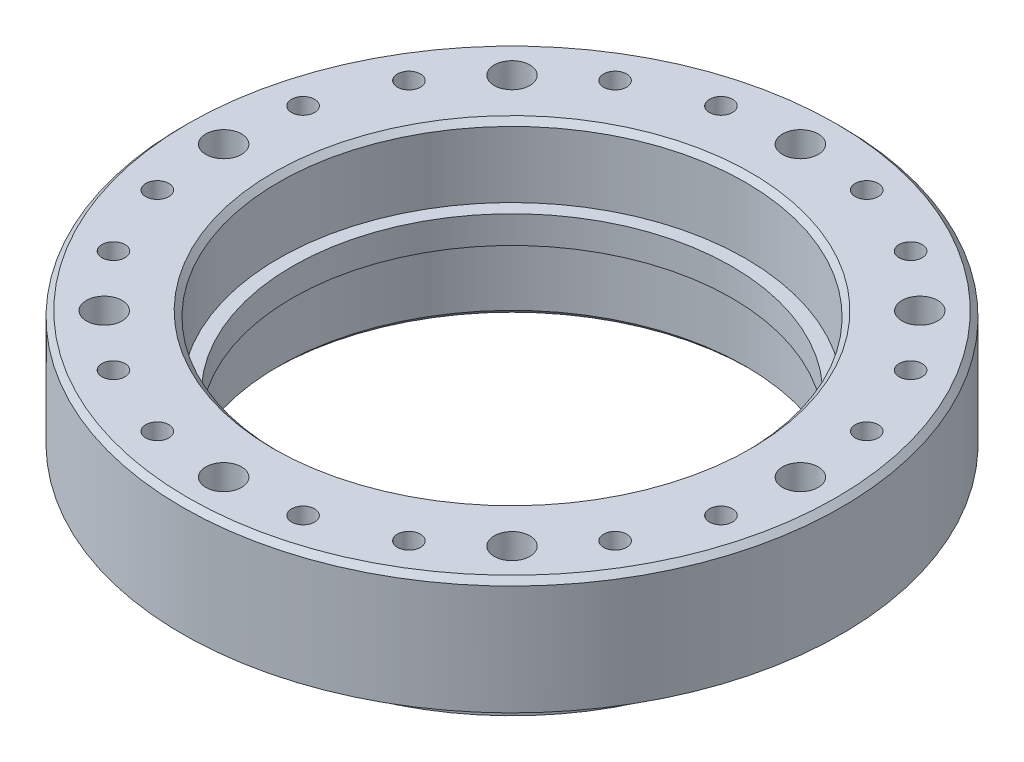
from build123d import *

# Parameters (mm, degrees)
SKETCH_1_R                = 60
SKETCH_1_R_2              = 40
EXTRUDE_1_DEPTH           = 15.5
CHAMFER_1_SIZE            = 1
HOLE_WIZARD_1_D           = 6.5
HOLE_WIZARD_1_CBORE_D     = 11
HOLE_WIZARD_1_CBORE_DEPTH = 6.8
SKETCH_7_R                = 42.5
CUT_EXTRUDE_2_DEPTH       = 13
CUT_EXTRUDE_START         = -13
SKETCH_8_R                = 42.5
CUT_EXTRUDE_3_DEPTH       = 13
SKETCH_9_R                = 67.994168063
SKETCH_9_R_2              = 46.5
CUT_EXTRUDE_4_DEPTH       = 10
HOLE_WIZARD_M5_1_D        = 4.2
PATTERN_CIRCULAR_1_COUNT  = 8
SKETCH_10_R               = 6
CUT_EXTRUDE_5_DEPTH       = 10
PATTERN_CIRCULAR_2_COUNT  = 2
PATTERN_CIRCULAR_2_ANGLE  = 45
PATTERN_CIRCULAR_3_COUNT  = 2
PATTERN_CIRCULAR_3_ANGLE  = 45
CHAMFER_2_SIZE            = 1


with BuildPart() as part:
    # 草图1 → 凸台-拉伸1 (new, symmetric)
    with BuildSketch(Plane(origin=(0, 0, 0), x_dir=(1, 0, 0), z_dir=(0, 1, 0))):
        with Locations(Location((0, 0, 0), (0, 0, 270))):
            Circle(SKETCH_1_R)
        with Locations(Location((0, 0, 0), (0, 0, 270))):
            Circle(SKETCH_1_R_2, mode=Mode.SUBTRACT)
    extrude(amount=EXTRUDE_1_DEPTH, both=True)

    # 倒角1
    chamfer_1_edges = [part.edges().sort_by_distance(p)[0] for p in [
        (0, -15.5, -60),
        (0, 15.5, -60),
        (0, -15.5, -40),
        (0, 15.5, -40),
    ]]
    chamfer(chamfer_1_edges, length=CHAMFER_1_SIZE)

    # 打孔尺寸根据内六角圆柱头螺钉的类型1 (through all)
    with Locations(Plane(origin=(-41.126423616, -15.5, 15.006070464), x_dir=(1, 0, 0), z_dir=(0, -1, 0))):
        with Locations((-11.373576384, -15.006070464), (93.626423616, -15.006070464), (41.126423616, -67.506070464), (41.126423616, 37.493929536)):
            hole_wizard_1 = CounterBoreHole(HOLE_WIZARD_1_D / 2, HOLE_WIZARD_1_CBORE_D / 2, HOLE_WIZARD_1_CBORE_DEPTH)

    # 草图7 → 切除-拉伸2 (cut)
    with BuildSketch(Plane(origin=(0, 15.5, 0), x_dir=(1, 0, 0), z_dir=(0, 1, 0))):
        with Locations(Location((0, 0, 0), (0, 0, 270))):
            Circle(SKETCH_7_R)
    extrude(amount=-CUT_EXTRUDE_2_DEPTH, mode=Mode.SUBTRACT)

    # 草图8 → 切除-拉伸3 (cut)
    with BuildSketch(Plane.XZ.offset(15.5).offset(CUT_EXTRUDE_START)):
        with Locations(Location((0, 0, 0), (0, 0, 90))):
            Circle(SKETCH_8_R)
    extrude(amount=CUT_EXTRUDE_3_DEPTH, mode=Mode.SUBTRACT)

    # 草图9 → 切除-拉伸4 (cut)
    with BuildSketch(Plane.XZ.offset(15.5)):
        Circle(SKETCH_9_R)
        with Locations(Location((0, 0, 0), (0, 0, 270))):
            Circle(SKETCH_9_R_2, mode=Mode.SUBTRACT)
    extrude(amount=-CUT_EXTRUDE_4_DEPTH, mode=Mode.SUBTRACT)

    # M5 螺纹孔1 (through all)
    with Locations(Plane(origin=(22.072004657, -5.5, -2.458986171), x_dir=(-1, 0, 0), z_dir=(0, -1, 0))):
        with Locations((-23.594340847, 24.440547066), (-29.239820284, 10.811154044)):
            hole_wizard_m5_1 = Hole(HOLE_WIZARD_M5_1_D / 2)

    # 阵列(圆周)1: M5 螺纹孔1 ×8 about axis
    pattern_circular_1_axis = Axis((0, 0, 0), (0, 1, 0))
    for i in range(1, PATTERN_CIRCULAR_1_COUNT):
        add(hole_wizard_m5_1.rotate(pattern_circular_1_axis, i * 360 / PATTERN_CIRCULAR_1_COUNT), mode=Mode.SUBTRACT)

    # 草图10 → 切除-拉伸5 (cut)
    with BuildSketch(Plane.XZ.offset(5.5)):
        with Locations(Location((0, -52.5, 0), (0, 0, 270))):
            Circle(SKETCH_10_R)
        with Locations(Location((52.5, 0, 0), (0, 0, 270))):
            Circle(SKETCH_10_R)
        with Locations(Location((0, 52.5, 0), (0, 0, 270))):
            Circle(SKETCH_10_R)
        with Locations(Location((-52.5, 0, 0), (0, 0, 270))):
            Circle(SKETCH_10_R)
    cut_extrude_5 = extrude(amount=-CUT_EXTRUDE_5_DEPTH, mode=Mode.SUBTRACT)

    # 阵列(圆周)2: 打孔尺寸根据内六角圆柱头螺钉的类型1 ×2 about axis
    pattern_circular_2_axis = Axis((0, 0, 0), (0, -1, 0))
    for i in range(1, PATTERN_CIRCULAR_2_COUNT):
        add(hole_wizard_1.rotate(pattern_circular_2_axis, i * PATTERN_CIRCULAR_2_ANGLE / (PATTERN_CIRCULAR_2_COUNT - 1)), mode=Mode.SUBTRACT)

    # 阵列(圆周)3: 切除-拉伸5 ×2 about axis
    pattern_circular_3_axis = Axis((0, 0, 0), (0, -1, 0))
    for i in range(1, PATTERN_CIRCULAR_3_COUNT):
        add(cut_extrude_5.rotate(pattern_circular_3_axis, i * PATTERN_CIRCULAR_3_ANGLE / (PATTERN_CIRCULAR_3_COUNT - 1)), mode=Mode.SUBTRACT)

    # 倒角2
    chamfer_2_edges = [part.edges().sort_by_distance(p)[0] for p in [
        (0, 15.5, -42.5),
        (0, -15.5, -42.5),
    ]]
    chamfer(chamfer_2_edges, length=CHAMFER_2_SIZE)


solid = part.part
